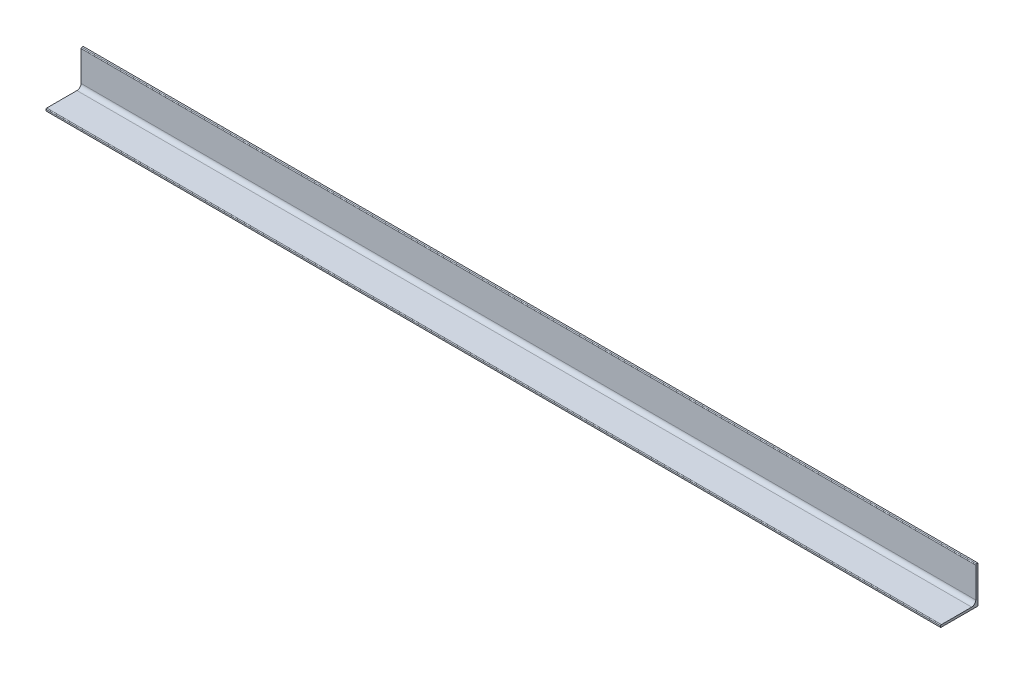
SolidWorks part; units mm, degrees
ref_plane "Front" through (0, 0, 0) normal (0, 0, 1) x (1, 0, 0)
ref_plane "Top" through (0, 0, 0) normal (0, 1, 0) x (1, 0, 0)
ref_plane "Right" through (0, 0, 0) normal (1, 0, 0) x (0, 0, -1)
sketch "Sketch1" plane through (0, 0, 0) normal (1, 0, 0) x (0, 1, 0)
  line L0 (0, 50) -> (0, 0)
  line L1 (0, 0) -> (50, 0)
  line L2 (3, 49) -> (3, 8.5)
  line L3 (8.5, 3) -> (49, 3)
  line L4 (0, 50) -> (2, 50)
  line L5 (50, 0) -> (50, 2)
  arc A0 (2, 50) -> (3, 49) centre (2, 49) cw
  arc A1 (50, 2) -> (49, 3) centre (49, 2) ccw
  arc A2 (3, 8.5) -> (8.5, 3) centre (8.5, 8.5) ccw
extrude "Base" add sketch "Sketch1" along normal blind 1200
equation "\"r1@Sketch1\" = \"d@Sketch1\" / 3"
equation "\"d1@Sketch1\" = \"d@Sketch1\""
equation "\"b1@Sketch1\" = \"b@Sketch1\""
